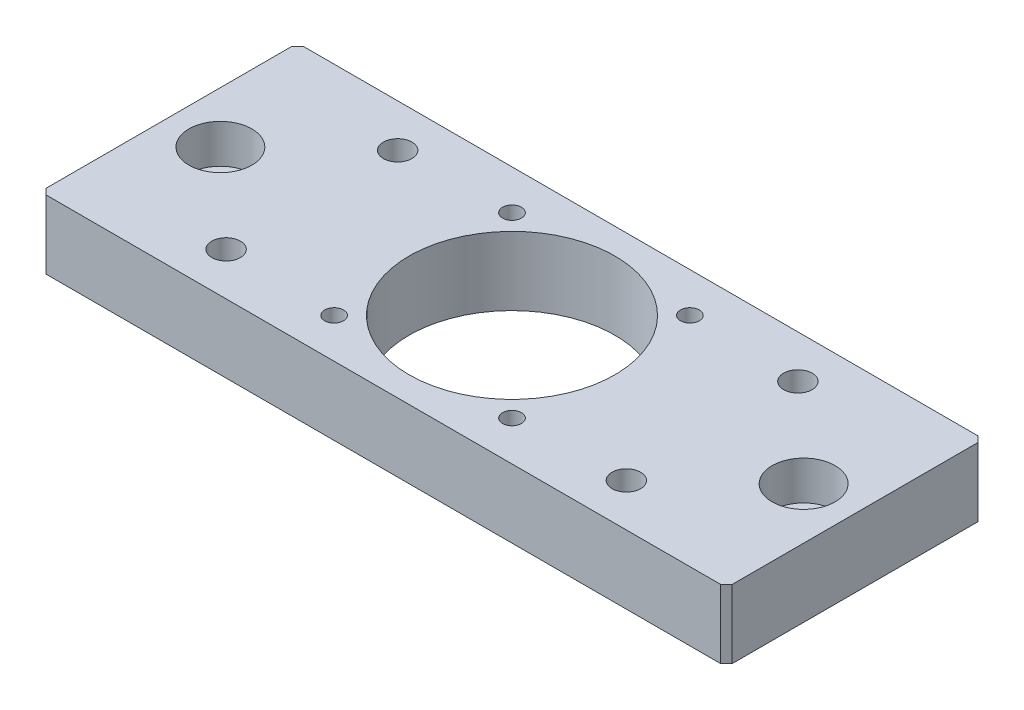
SolidWorks part; units mm, degrees
material "S45C"
ref_plane "Front Plane" through (0, 0, 0) normal (0, 0, 1) x (1, 0, 0)
ref_plane "Top Plane" through (0, 0, 0) normal (0, 1, 0) x (1, 0, 0)
ref_plane "Right Plane" through (0, 0, 0) normal (1, 0, 0) x (0, 0, -1)
sketch "Sketch1" plane through (0, 0, 0) normal (0, 1, 0) x (1, 0, 0)
  line L1 (60, 22.5) -> (-60, 22.5)
  line L2 (60, 22.5) -> (60, -22.5)
  line L3 (60, -22.5) -> (-60, -22.5)
  line L4 (-60, 22.5) -> (-60, -22.5)
  line L5 (60, 22.5) -> (-60, -22.5) construction
  line L6 (60, -22.5) -> (-60, 22.5) construction
  point P0 (0, 0)
  dimension "D1" = 45
  dimension "D2" = 120
extrude "Boss-Extrude1" add sketch "Sketch1" along normal blind 12
chamfer "Chamfer1" distance 1 angle 45 4 edges at (60, 6, -22.5) (60, 6, 22.5) (-60, 6, -22.5) (-60, 6, 22.5)
sketch "Sketch2" plane through (0, 12, 0) normal (0, 1, 0) x (1, 0, 0)
  circle A0 centre (0, 0) radius 18
  dimension "D1" = 36
extrude "Cut-Extrude1" cut sketch "Sketch2" against normal through all
hole_wizard "M4 Tapped Hole1" positions "Sketch4" profile "Sketch3" tap size "M4" standard "ISO" end condition through all
sketch "Sketch4" plane through (0, 12, 0) normal (0, 1, 0) x (-1, 0, 0)
  line L0 (0, 0) -> (0, -7.7454) construction
  line L2 (0, 0) -> (-9.3921, 0) construction
  point P1 (15.5565, -15.5565)
  point P15 (15.5565, 15.5565)
  point P16 (-15.5565, 15.5565)
  point P17 (-15.5565, -15.5565)
  dimension "D1" = 31.113
  dimension "D2" = 31.113
sketch "Sketch3" plane through (-15.5565, 12, -15.5565) normal (1, 0, 0) x (0, 0, 1)
  line L0 (0, 0) -> (0, 12)
  line L1 (0, 12) -> (1.65, 12)
  line L2 (1.65, 12) -> (1.65, 0)
  line L5 (1.65, 0) -> (0, 0)
  line L11 (0, -6.35) -> (0, 107.95) construction
  dimension "通孔螺纹孔钻头直径" = 3.3
  dimension "通孔螺纹孔钻头深度" = 12
cosmetic thread "Cosmetic Thread1" parameters "D2"=4
cosmetic thread "Cosmetic Thread2" parameters "D2"=4
cosmetic thread "Cosmetic Thread3" parameters "D2"=4
cosmetic thread "Cosmetic Thread4" parameters "D2"=4
hole_wizard "Hole size per socket head cap screw type1" positions "Sketch6" profile "Sketch5" counterbore size "M6" standard "GB" end condition through all
sketch "Sketch6" plane through (0, 12, 0) normal (0, 1, 0) x (-1, 0, 0)
  line L0 (0, 0) -> (0, 8.4773) construction
  point P0 (51, 0)
  point P8 (-51, 0)
  dimension "D1" = 102
sketch "Sketch5" plane through (-51, 12, 0) normal (1, 0, 0) x (0, 0, 1)
  line L0 (0, 0) -> (0, 12)
  line L1 (0, 12) -> (3.3, 12)
  line L3 (3.3, 12) -> (3.3, 6.8)
  line L4 (3.3, 6.8) -> (5.5, 6.8)
  line L5 (5.5, 6.8) -> (5.5, 0)
  line L7 (5.5, 0) -> (0, 0)
  line L11 (0, -6.35) -> (0, 107.95) construction
  dimension "通孔孔直径" = 6.6
  dimension "通孔孔深度" = 12
  dimension "柱形沉头孔直径" = 11
  dimension "柱形沉头孔深度" = 6.8
sketch "Sketch7" plane through (0, 0, 0) normal (0, -1, 0) x (1, 0, 0)
  circle A0 centre (51, 0) radius 6
  circle A1 centre (-51, 0) radius 6
  dimension "D1" = 12
extrude "Cut-Extrude2" cut sketch "Sketch7" against normal blind 3.2
hole_wizard "M4 Tapped Hole2" positions "Sketch9" profile "Sketch8" tap size "M4" standard "ISO"
sketch "Sketch9" plane through (0, 0, -22.5) normal (0, 0, -1) x (-1, 0, 0)
  point P0 (-27.5, 7)
sketch "Sketch8" plane through (27.5, 7, -22.5) normal (1, 0, 0) x (0, 1, 0)
  line L0 (0, 0) -> (0, 12.4914)
  line L1 (0, 12.4914) -> (1.65, 11.5)
  line L2 (1.65, 11.5) -> (1.65, 0)
  line L5 (1.65, 0) -> (0, 0)
  line L10 (0, 12.4914) -> (-1.65, 11.5) construction
  line L11 (0, -6.35) -> (0, 107.95) construction
  dimension "螺纹孔钻头直径" = 3.3
  dimension "螺纹孔钻头深度" = 11.5
  dimension "导头角度" = 118
cosmetic thread "Cosmetic Thread5"
hole_wizard "M6 Tapped Hole1" positions "Sketch10" profile "Sketch11" tap size "M6" standard "GB" end condition up to next
sketch "Sketch10" plane through (0, 12, 0) normal (0, 1, 0) x (1, 0, 0)
  line L1 (0, 0) -> (0, -7.3507) construction
  line L3 (0, 0) -> (-7.7742, 0) construction
  point P0 (35, -15)
  point P2 (35, 15)
  point P4 (-35, -15)
  point P6 (-35, 15)
  dimension "D1" = 70
  dimension "D2" = 30
sketch "Sketch11" plane through (35, 12, 15) normal (1, 0, 0) x (0, 0, 1)
  line L0 (0, 0) -> (0, 12)
  line L1 (0, 12) -> (2.5, 12)
  line L2 (2.5, 12) -> (2.5, 0)
  line L5 (2.5, 0) -> (0, 0)
  line L11 (0, -6.35) -> (0, 107.95) construction
  dimension "通孔螺纹孔钻头直径" = 5
  dimension "通孔螺纹孔钻头深度" = 12
cosmetic thread "Cosmetic Thread6"
cosmetic thread "Cosmetic Thread7"
cosmetic thread "Cosmetic Thread8"
cosmetic thread "Cosmetic Thread9"
